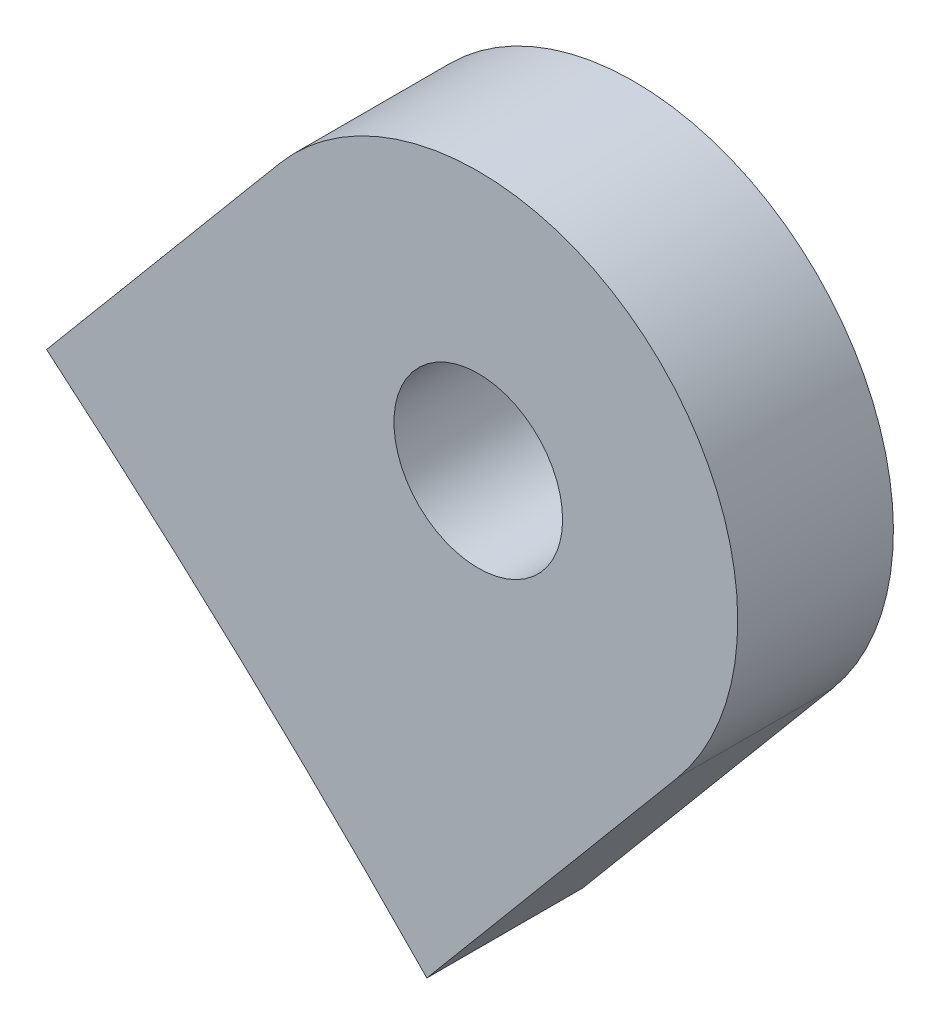
SolidWorks part; units mm, degrees
material "钢板12/Q235A"
ref_plane "Front Plane" through (0, 0, 0) normal (0, 0, 1) x (1, 0, 0)
ref_plane "Top Plane" through (0, 0, 0) normal (0, 1, 0) x (1, 0, 0)
ref_plane "Right Plane" through (0, 0, 0) normal (1, 0, 0) x (0, 0, -1)
sketch "Sketch1" plane through (0, 0, 0) normal (0, 0, 1) x (1, 0, 0)
  line L0 (0, 0) -> (0, 387.5) construction
  line L1 (0, 0) -> (249.0802, 296.8422) construction
  line L2 (249.0802, 296.8422) -> (267.0332, 318.2378)
  line L3 (278.3914, 269.545) -> (297.675, 292.5263)
  line L4 (282.3541, 305.3821) -> (264.0887, 283.5726) construction
  circle A0 centre (0, 0) radius 387.5 construction
  arc A1 (267.0332, 318.2378) -> (297.675, 292.5263) centre (282.3541, 305.3821) cw
  arc A2 (249.0802, 296.8422) -> (278.3914, 269.545) centre (0, 0) cw
  circle A3 centre (282.3541, 305.3821) radius 6.5
  dimension "D1" = 775
  dimension "D3" = 20
  dimension "D5" = 13
  dimension "D2" = 40
  dimension "D4" = 30
  dimension "D6" = 40
extrude "Boss-Extrude1" add sketch "Sketch1" along normal mid plane 12
